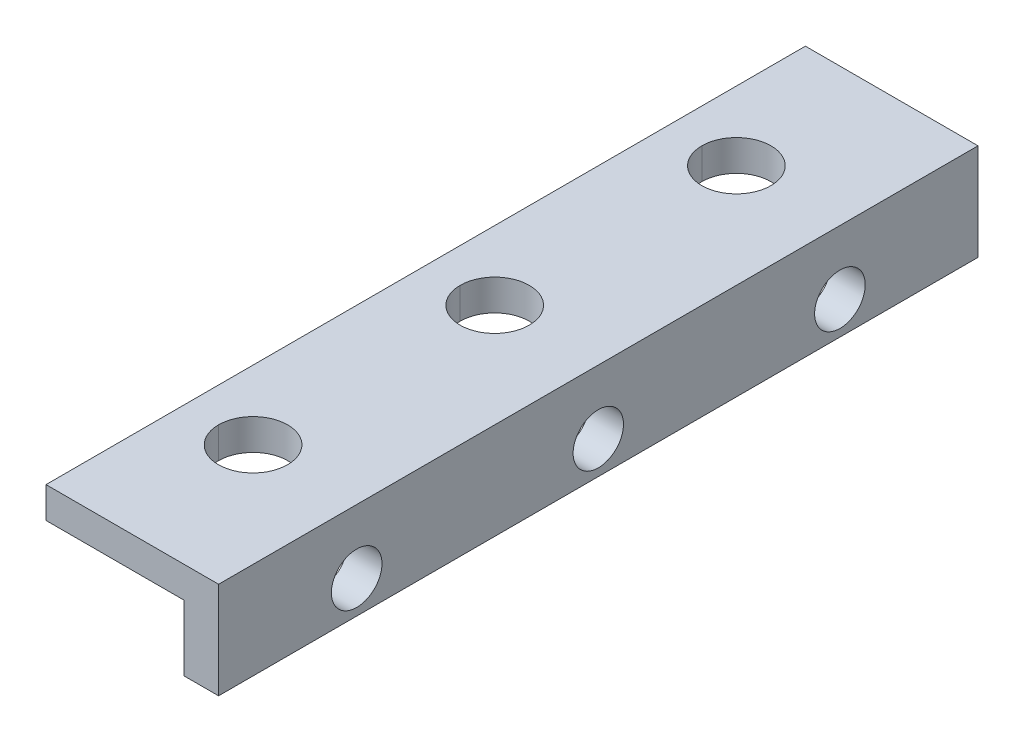
from build123d import *

# Parameters (mm, degrees)
EXTRUDE_1_DEPTH     = 220
SKETCH_2_R          = 10
CUT_EXTRUDE_1_DEPTH = 24
SKETCH_3_R          = 10
CUT_EXTRUDE_2_DEPTH = 24
SKETCH_4_R          = 7.332886018
SKETCH_4_R_2        = 7.301331484
SKETCH_4_R_3        = 6.603217824
CUT_EXTRUDE_3_DEPTH = 10
CUT_EXTRUDE_START   = -45
SKETCH_5_R          = 7.332886018
SKETCH_5_R_2        = 7.301331484
SKETCH_5_R_3        = 6.603217824
CUT_EXTRUDE_4_DEPTH = 45


with BuildPart() as part:
    # 草图1 → 凸台-拉伸1 (new body)
    with BuildSketch(Plane.XY):
        Polygon((-55.555555556, 26.25), (-5.555555556, 26.25), (-5.555555556, -1.75), (-15.555555556, -1.75), (-15.555555556, 17.25), (-55.555555556, 17.25), align=None)
    extrude(amount=EXTRUDE_1_DEPTH)

    # 草图2 → 切除-拉伸1 (cut)
    with BuildSketch(Plane(origin=(982.792188559, 17.25, -600.126281628), x_dir=(0.9997402704834758, 0, 0.022790163966647386), z_dir=(0, -1, 0))):
        with Locations(Location((-1000.30321436, 803.168334002, 0), (0, 0, 358.694106729))):
            Circle(SKETCH_2_R)
        with Locations(Location((-1001.898940295, 733.168334002, 0), (0, 0, 358.694106729))):
            Circle(SKETCH_2_R)
        with Locations(Location((-1003.49466623, 663.168334002, 0), (0, 0, 358.694106729))):
            Circle(SKETCH_2_R)
        with Locations((-915.325705826, 801.212988999)):
            Circle(SKETCH_2_R)
        with Locations((-916.921431761, 731.212988999)):
            Circle(SKETCH_2_R)
        with Locations((-918.516743239, 661.231170065)):
            Circle(SKETCH_2_R)
    extrude(amount=-CUT_EXTRUDE_1_DEPTH, mode=Mode.SUBTRACT)

    # 草图3 → 切除-拉伸2 (cut)
    with BuildSketch(Plane(origin=(-968.90329967, 17.25, 820.126281628), x_dir=(-0.9997402704834758, 0, -0.022790163966647077), z_dir=(0, -1, 0))):
        with Locations((-1000.30321436, 803.168334002)):
            Circle(SKETCH_3_R)
        with Locations((-1001.898940295, 733.168334002)):
            Circle(SKETCH_3_R)
        with Locations((-1003.49466623, 663.168334002)):
            Circle(SKETCH_3_R)
        with Locations((-915.325705826, 801.212988999)):
            Circle(SKETCH_3_R)
        with Locations((-916.921431761, 731.212988999)):
            Circle(SKETCH_3_R)
        with Locations((-918.516743239, 661.231170065)):
            Circle(SKETCH_3_R)
    extrude(amount=-CUT_EXTRUDE_2_DEPTH, mode=Mode.SUBTRACT)

    # 草图4 → 切除-拉伸3 (cut)
    with BuildSketch(Plane(origin=(-15.555555556, -796.892477777, -600.126281629), x_dir=(0, -1, 0), z_dir=(-1, 0, 0))):
        with Locations(Location((-804.642477777, 640.126281628, 0), (0, 0, 90))):
            Circle(SKETCH_4_R)
        with Locations(Location((-804.642477777, 710.126281628, 0), (0, 0, 90))):
            Circle(SKETCH_4_R_2)
        with Locations(Location((-804.642477777, 780.126281628, 0), (0, 0, 90))):
            Circle(SKETCH_4_R_3)
    extrude(amount=-CUT_EXTRUDE_3_DEPTH, mode=Mode.SUBTRACT)

    # 草图5 → 切除-拉伸4 (cut)
    with BuildSketch(Plane(origin=(29.444444444, -796.892477777, 820.126281629), x_dir=(0, -1, 0), z_dir=(1, 0, 0)).offset(CUT_EXTRUDE_START)):
        with Locations(Location((-804.642477777, 640.126281628, 0), (0, 0, 90))):
            Circle(SKETCH_5_R)
        with Locations(Location((-804.642477777, 710.126281628, 0), (0, 0, 270))):
            Circle(SKETCH_5_R_2)
        with Locations((-804.642477777, 780.126281628)):
            Circle(SKETCH_5_R_3)
    extrude(amount=CUT_EXTRUDE_4_DEPTH, mode=Mode.SUBTRACT)


solid = part.part
